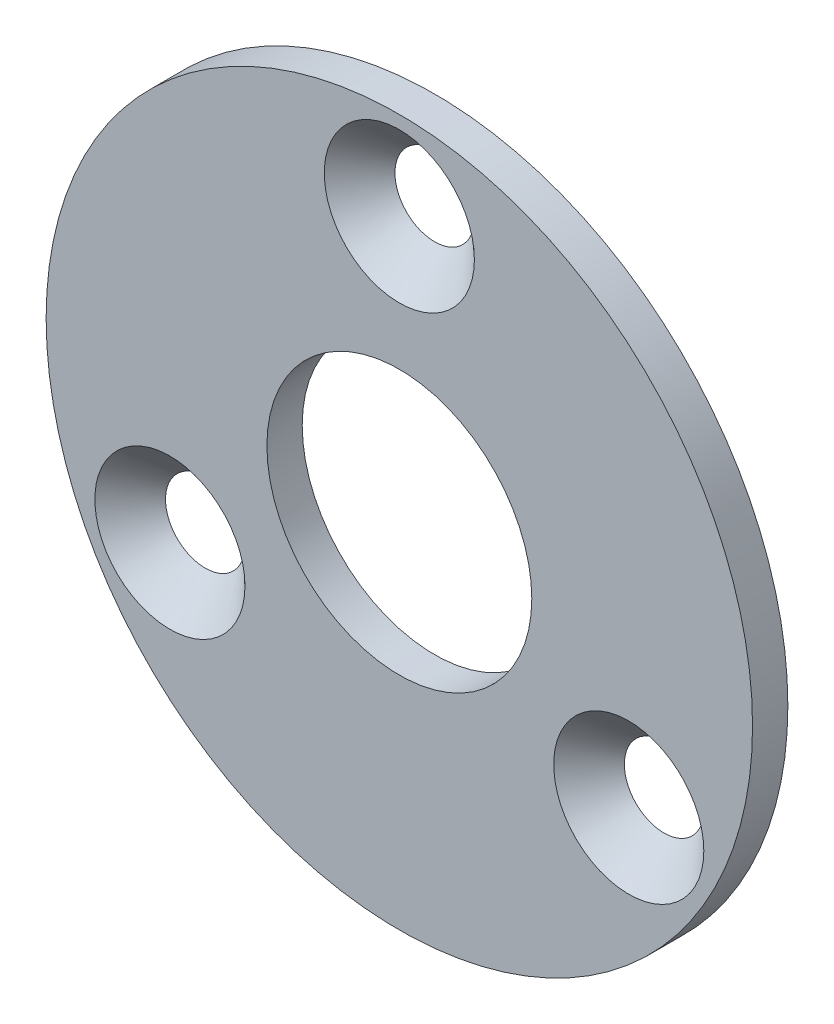
SolidWorks part; units mm, degrees
ref_plane "Front Plane" through (0, 0, 0) normal (0, 0, 1) x (1, 0, 0)
ref_plane "Top Plane" through (0, 0, 0) normal (0, 1, 0) x (1, 0, 0)
ref_plane "Right Plane" through (0, 0, 0) normal (1, 0, 0) x (0, 0, -1)
other "Configuration Table"
sketch "Sketch1" plane through (0, 0, 0) normal (1, 0, 0) x (0, 0, -1)
  line L0 (-4.3667, 0) -> (12.9667, 0) construction
  line L1 (0, 20) -> (0, 7.5)
  line L2 (0, 7.5) -> (2, 7.5)
  line L3 (2, 7.5) -> (2, 20)
  line L4 (2, 20) -> (0, 20)
  dimension "D1" = 2
  dimension "D2" = 7.5
  dimension "D3" = 20
revolve "Revolve1" add sketch "Sketch1" angle 360 about L0
sketch "Sketch2" plane through (0, 0, 0) normal (1, 0, 0) x (0, 0, -1)
  line L0 (-4.9082, 0) -> (16.9855, 0) construction
  line L1 (0, 19.25) -> (2, 17.25)
  line L2 (0, 20) -> (0, -20) construction
  line L3 (2, -20) -> (2, 20) construction
  line L4 (2, 17.25) -> (2, 15)
  line L6 (0, 15) -> (0, 19.25)
  line L7 (0, 15) -> (2, 15)
  line L8 (-0.9092, 15) -> (3.6137, 15) construction
  dimension "D1" = 15
  dimension "D2" = 2.25
  dimension "D3" = 45
  dimension "D4" = 2
revolve "Cut-Revolve1" cut sketch "Sketch2" angle 360 about L8
pattern_circular "CirPattern1" count 3 over 360 about axis through (0, 0, 0) along (0, 0, 1) of "Cut-Revolve1"
